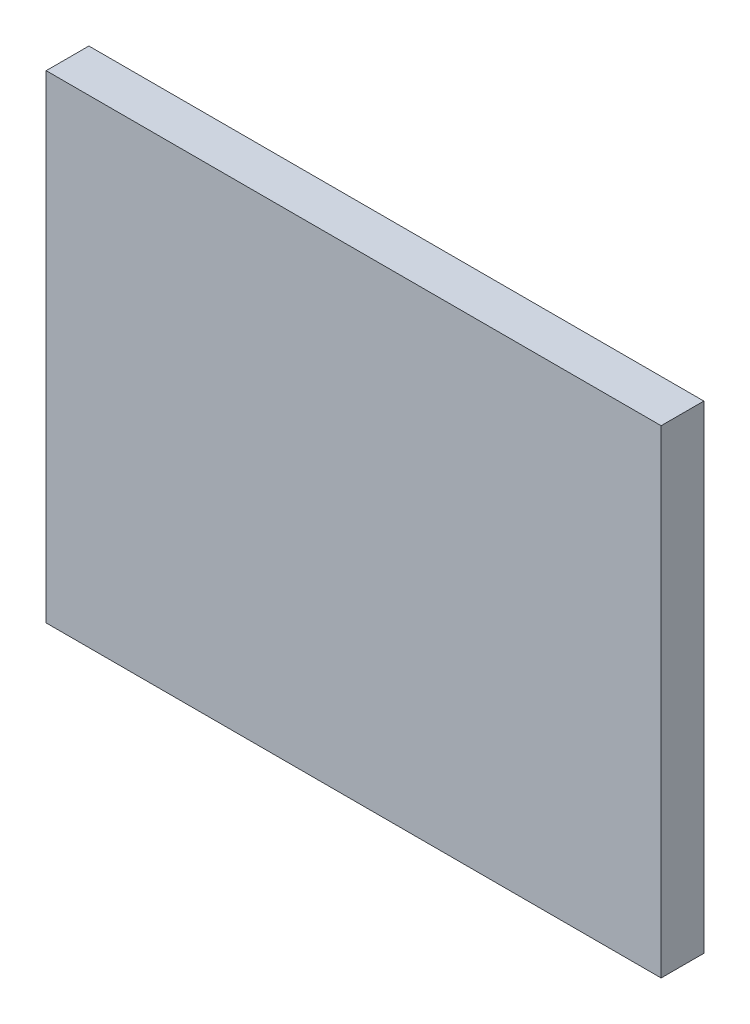
from build123d import *

# Parameters (mm, degrees)
SKETCH_1_W      = 360
SKETCH_1_H      = 280
EXTRUDE_1_DEPTH = 25


with BuildPart() as part:
    # 草图1 → 凸台-拉伸1 (new body)
    with BuildSketch(Plane.XY):
        Rectangle(SKETCH_1_W, SKETCH_1_H)
    extrude(amount=EXTRUDE_1_DEPTH)


solid = part.part
